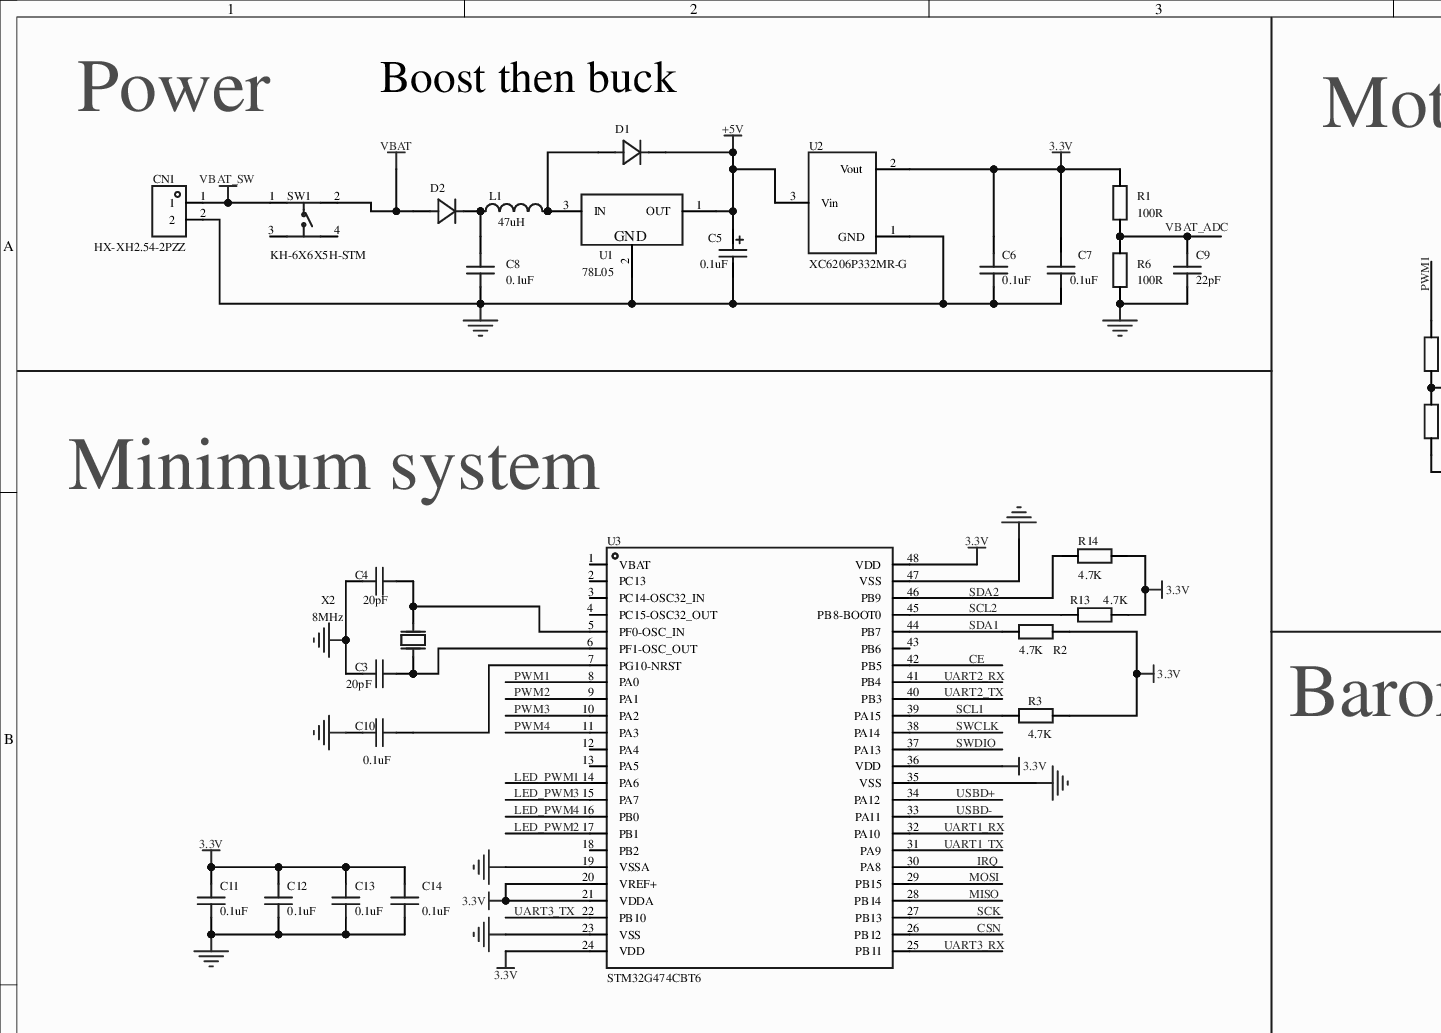
[diagram p0: MISC51791-2.schdoc, top left]
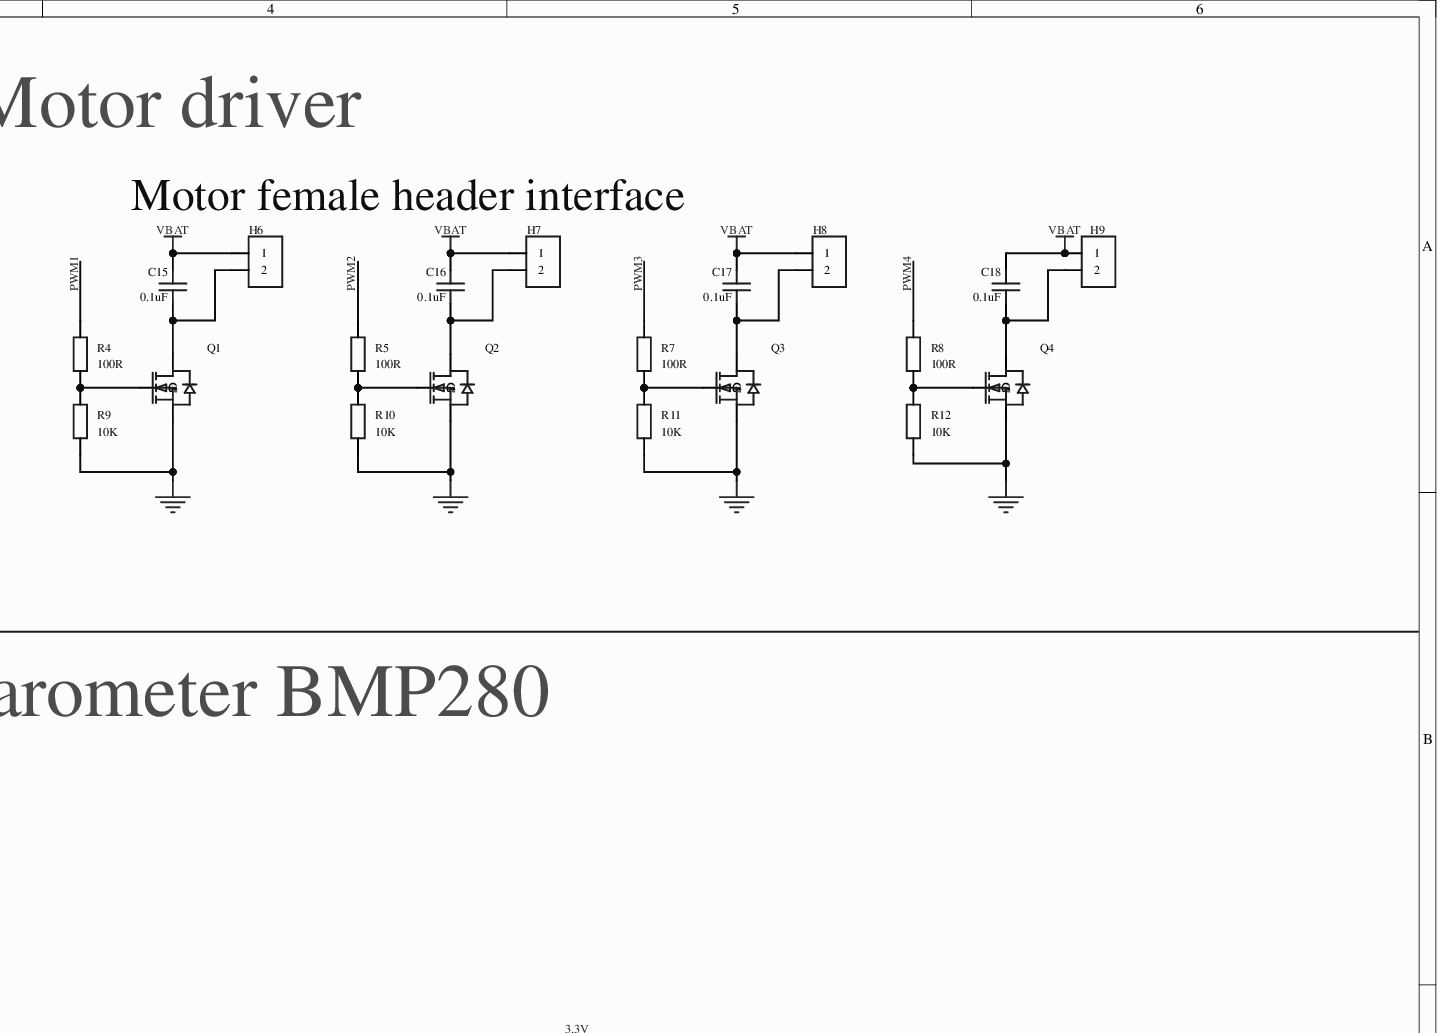
[diagram p1: MISC51791-2.schdoc, top right]
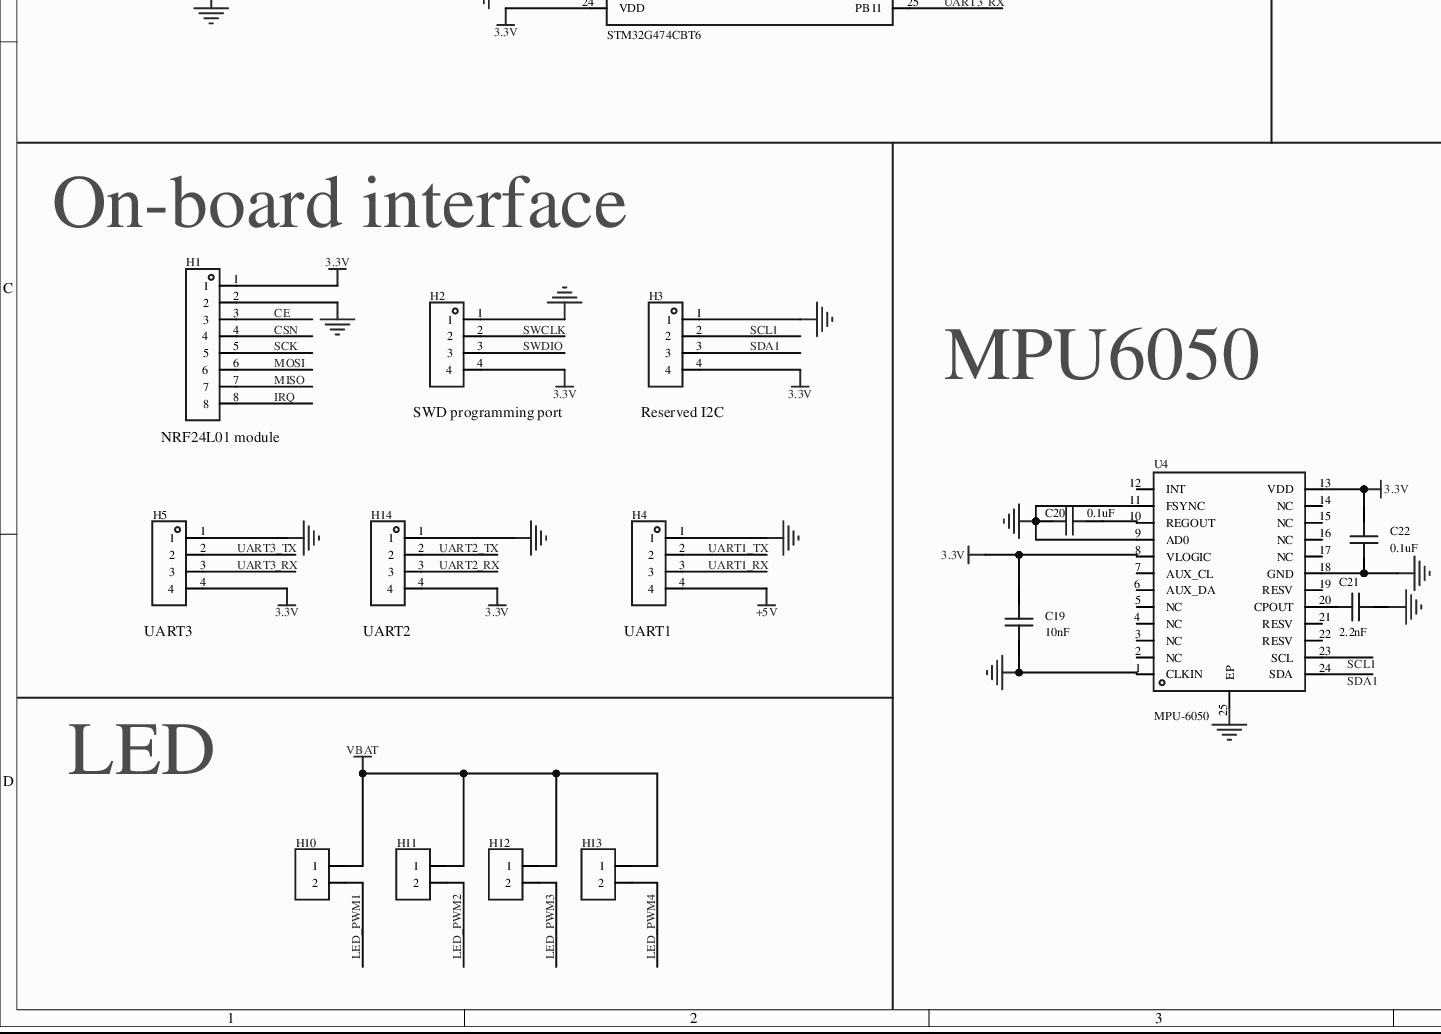
[diagram p2: MISC51791-2.schdoc, bottom left]
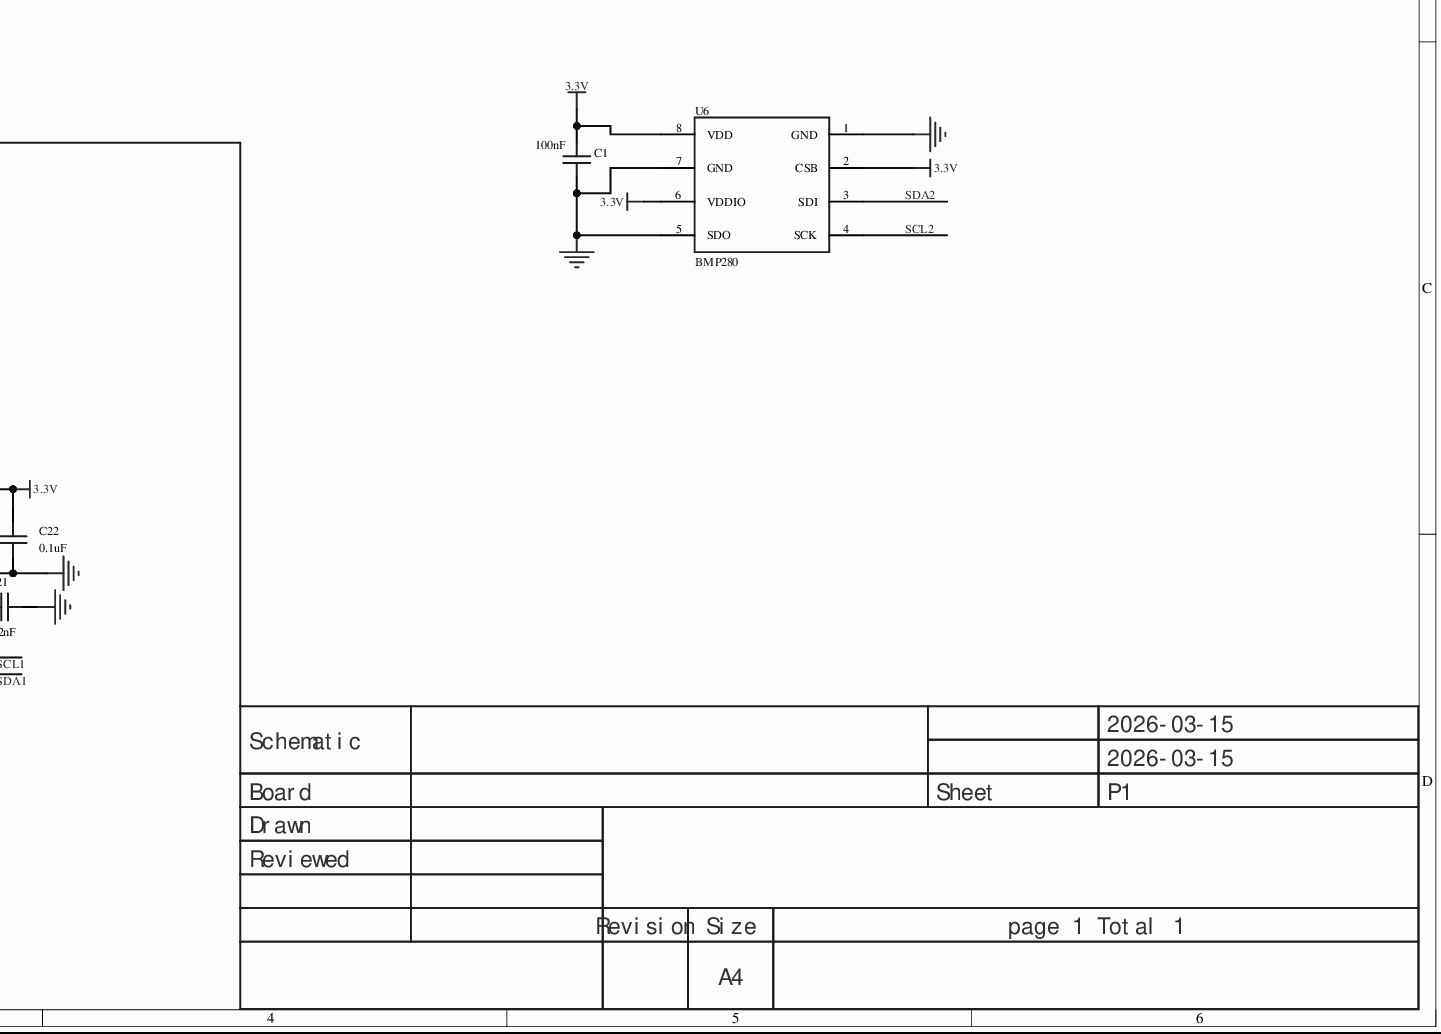
[diagram p3: MISC51791-2.schdoc, bottom right]
# Altium project MISC51791-3.PrjPcb
1 sheet, 64 parts. Net scope: global (net labels, ports and power ports of the same name join across sheets).
Board file: MISC51791.pcbdoc

## Sheet MISC51791-2.schdoc
size 420 x 297 mm; Version: V1.0; @Project Name: MISC51791; @Update Date: 2026-03-15; @Create Date: 2026-03-15; @Board Name: MISC51791; @Create Time: 18:26:02; @Page Count: 1; @Page No: 1; @Schematic Name: MISC51791; @Update Time: 18:26:02; Size: A4

### Parts
C1  100nF  [C0603]
C3  20pF  [C0603]
C4  20pF  [C0603]
C5  0.1uF  [C_Ele_SMD_3x5.4mm]
C6  0.1uF  [C0603]
C7  0.1uF  [C0603]
C8  0.1uF  [C0603]
C9  22pF  [C0603]
C10  0.1uF  [C0603]
C11  0.1uF  [C0603]
C12  0.1uF  [C0603]
C13  0.1uF  [C0603]
C14  0.1uF  [C0603]
C15  0.1uF  [C0603]
C16  0.1uF  [C0603]
C17  0.1uF  [C0603]
C18  0.1uF  [C0603]
C19  10nF  [C0603]
C20  0.1uF  [C0603]
C21  2.2nF  [C0603]
C22  0.1uF  [C0603]
CN1  HX-XH2.54-2PZZ  [CONN-TH_2P-P2.50_HX-2.54MM-2P-ZZ-MS]
D1  (no value)  [DO_1N4007]
D2  (no value)  [DO_1N4007]
H1  (no value)  [HDR-TH_8P-P2.54-V-F-1]
H2  (no value)  [HDR-TH_4P-P2.54-V-F]
H3  (no value)  [HDR-TH_4P-P2.54-V-F]
H4  (no value)  [HDR-TH_4P-P2.54-V-F]
H5  (no value)  [HDR-TH_4P-P2.54-V-F]
H6  (no value)  [HDR-TH_2P-P2.54-V-F]
H7  (no value)  [HDR-TH_2P-P2.54-V-F]
H8  (no value)  [HDR-TH_2P-P2.54-V-F]
H9  (no value)  [HDR-TH_2P-P2.54-V-F]
H10  (no value)  [HDR-TH_2P-P2.54-V-F]
H11  (no value)  [HDR-TH_2P-P2.54-V-F]
H12  (no value)  [HDR-TH_2P-P2.54-V-F]
H13  (no value)  [HDR-TH_2P-P2.54-V-F]
H14  (no value)  [HDR-TH_4P-P2.54-V-F]
L1  47uH  [L0603]
Q1  (no value)  [SOT-23-3_L2.9-W1.3-P1.90-LS2.4-BR]
Q2  (no value)  [SOT-23-3_L2.9-W1.3-P1.90-LS2.4-BR]
Q3  (no value)  [SOT-23-3_L2.9-W1.3-P1.90-LS2.4-BR]
Q4  (no value)  [SOT-23-3_L2.9-W1.3-P1.90-LS2.4-BR]
R1  100R  [R0603]
R2  4.7K  [R0603]
R3  4.7K  [R0603]
R4  100R  [R0603]
R5  100R  [R0603]
R6  100R  [R0603]
R7  100R  [R0603]
R8  100R  [R0603]
R9  10K  [R0603]
R10  10K  [R0603]
R11  10K  [R0603]
R12  10K  [R0603]
R13  4.7K  [R0603]
R14  4.7K  [R0603]
SW1  KH-6X6X5H-STM  [SW-SMD_4P-L6.0-W6.0-P4.50-LS9.0_H5.0]
U1  78L05  [SOT-89-3_L4.5-W2.5-P1.50-LS4.2-BR]
U2  XC6206P332MR-G  [SOT-23-3_L2.9-W1.6-P1.90-LS2.8-BR]
U3  STM32G474CBT6  [LQFP-48_L7.0-W7.0-P0.50-LS9.0-BL]
U4  MPU-6050  [QFN-24_L4.0-W4.0-P0.50-BL-EP2.7]
U6  BMP280  [LGA-8_L2.5-W2.0-P0.65_AMP6127]
X2  8MHz  [CRYSTAL-SMD_L5.0-W3.2]

### Nets
3.3V: C1.2 C6.2 C7.2 C11.2 C12.2 C13.2 C14.2 C19.2 C22.1 H1.1 H2.4 H3.4 H5.4 H14.4 R1.2 R2.2 R3.2 R13.2 R14.2 U2.2(Vout) U3.20(VREF+) U3.21(VDDA) U3.24(VDD) U3.36(VDD) U3.48(VDD) U4.8(VLOGIC) U4.13(VDD) U6.2(CSB) U6.6(VDDIO) U6.8(VDD)
+5V: C5.1 D1.1(K) H4.4 U1.1(OUT) U2.3(Vin)
GND: C1.1 C3.1 C4.1 C5.2 C6.1 C7.1 C8.1 C9.1 C10.1 C11.1 C12.1 C13.1 C14.1 C19.1 C20.1 C21.2 C22.2 CN1.2 H1.2 H2.1 H3.1 H4.1 H5.1 H14.1 Q1.2(S) Q2.2(S) Q3.2(S) Q4.2(S) R6.1 R9.1 R10.1 R11.1 R12.1 U1.2(GND) U2.1(GND) U3.19(VSSA) U3.23(VSS) U3.35(VSS) U3.47(VSS) U4.1(CLKIN) U4.9(AD0) U4.11(FSYNC) U4.18(GND) U4.25(EP) U6.1(GND) U6.5(SDO) U6.7(GND)
VBAT: C15.2 C16.2 C17.2 C18.2 D2.2(A) H6.1 H7.1 H8.1 H9.1 H10.1 H11.1 H12.1 H13.1 SW1.2
VBAT_SW: CN1.1 SW1.1
CE: H1.3 U3.42(PB5)
CSN: H1.4 U3.26(PB12)
IRQ: H1.8 U3.30(PA8)
LED_PWM1: H10.2 U3.14(PA6)
LED_PWM2: H11.2 U3.17(PB1)
LED_PWM3: H12.2 U3.15(PA7)
LED_PWM4: H13.2 U3.16(PB0)
MISO: H1.7 U3.28(PB14)
MOSI: H1.6 U3.29(PB15)
PWM1: R4.2 U3.8(PA0)
PWM2: R5.2 U3.9(PA1)
PWM3: R7.2 U3.10(PA2)
PWM4: R8.2 U3.11(PA3)
SCK: H1.5 U3.27(PB13)
SCL1: H3.2 R3.1 U3.39(PA15) U4.23(SCL)
SCL2: R13.1 U3.45(PB8-BOOT0) U6.4(SCK)
SDA1: H3.3 R2.1 U3.44(PB7) U4.24(SDA)
SDA2: R14.1 U3.46(PB9) U6.3(SDI)
SWCLK: H2.2 U3.38(PA14)
SWDIO: H2.3 U3.37(PA13)
UART1_RX: H4.3 U3.32(PA10)
UART1_TX: H4.2 U3.31(PA9)
UART2_RX: H14.3 U3.41(PB4)
UART2_TX: H14.2 U3.40(PB3)
UART3_RX: H5.3 U3.25(PB11)
UART3_TX: H5.2 U3.22(PB10)
USBD+: U3.34(PA12)
USBD-: U3.33(PA11)
NetC3_2: C3.2 U3.6(PF1-OSC_OUT) X2.1(OSC1)
NetC4_2: C4.2 U3.5(PF0-OSC_IN) X2.2(OSC2)
NetC8_2: C8.2 D2.1(K) L1.1
NetC9_2: C9.2 R1.1 R6.2
NetC10_2: C10.2 U3.7(PG10-NRST)
NetC15_1: C15.1 H6.2 Q1.3(D)
NetC16_1: C16.1 H7.2 Q2.3(D)
NetC17_1: C17.1 H8.2 Q3.3(D)
NetC18_1: C18.1 H9.2 Q4.3(D)
NetC20_2: C20.2 U4.10(REGOUT)
NetC21_1: C21.1 U4.20(CPOUT)
NetD1_2: D1.2(A) L1.2 U1.3(IN)
NetQ1_1: Q1.1(G) R4.1 R9.2
NetQ2_1: Q2.1(G) R5.1 R10.2
NetQ3_1: Q3.1(G) R7.1 R11.2
NetQ4_1: Q4.1(G) R8.1 R12.2

Not connected (* = marked no-connect by the designer): SW1 3* 4*; U3 1(VBAT)* 2(PC13)* 3(PC14-OSC32_IN)* 4(PC15-OSC32_OUT)* 12(PA4)* 13(PA5)* 18(PB2)* 43(PB6)*; U4 2(NC)* 3(NC)* 4(NC)* 5(NC)* 6(AUX_DA)* 7(AUX_CL)* 12(INT)* 14(NC)* 15(NC)* 16(NC)* 17(NC)* 19(RESV)* 21(RESV)* 22(RESV)*

### Notes on the sheet
- Power
- (near D1) Boost then buck
- Motor driver
- Motor female header interface
- Minimum system
- Barometer BMP280
- (near H1) On-board interface
- MPU6050
- (near H1) NRF24L01 module
- (near H2) SWD programming port
- (near H3) Reserved I2C
- (near H5) UART3
- (near H14) UART2
- (near H4) UART1
- LED
- Labels drawn without touching a wire or pin: VBAT_ADC
- 2026-03-15
- Schematic
- Board
- Sheet
- P1
- Drawn
- Reviewed
- Revision
- Size
- A4
- page 1 Total 1

### Library data of the parts
C1 C3 C4 C6-C22 = CAP_0603: Symbol: Capacitance; 3D Model: ac125912035d415993ca9572d50418b10819f05c4eef4c71ace90d822a990e87; 3D Model Transform: 62.992,31.496,0,0,0,0,0,0,0; ConvertToPcb: yes; ModelName: C0603_L1.6-W0.8-H0.8; Device: CAP_0603; Supplier Footprint: 0603; AddInBom: yes; FootprintName: C0603
  C1: Value: 100nF
  C3 C4: Value: 20pF
  C6-C8 C10-C18 C20 C22: Value: 0.1uF
  C9: Value: 22pF
  C19: Value: 10nF
  C21: Value: 2.2nF
C5 = C_Ele_SMD_3x5.4mm: Symbol: CAP; 3D Model: 0132c3d3fdbf4fd987f710a97e7a5b5d; 3D Model Transform: 129.9,149.58,209.06,-90,0,0,0,0,0; AddInBom: yes; ModelName: CAP-SMD_BD3.0-L3.3-W3.3-H5.3; Device: C_Ele_SMD_3x5.4mm; Supplier Footprint: SMD,3x5.4mm; Value: 0.1uF; ConvertToPcb: yes; FootprintName: C_Ele_SMD_3x5.4mm
CN1 = HX-XH2.54-2PZZ: Pin structure: 1x2P; pitch: 2.54mm; mounting: through-hole; reference series: XH; total pins: 2P; rows: 1; pins per row: 2; row spacing: -; rated current: 3A; contact material: brass; contact plating: tin; operating temperature: -25℃~+85℃;; Manufacturer: hanxia(韩下); 3D Model: 1cafe43f43c04794b29c478db770ea2f; 3D Model Transform: 295.275,228.7397,0,0,0,0,0,-19.685,-137.795; Number of PINs Per Row: 2; Voltage Rating: 250V; Plastic Material: PA66; Flame Retardant Rating: UL94V-0; AddInBom: yes; Symbol: HX-XH2.54-2PZZ; Device: HX-XH2.54-2PZZ; LCSC Part Name: 1x2P 间距:2.5mm 直插 系列:XH; Supplier Part: C42391660; Manufacturer Part: HX-XH2.54-2PZZ; Supplier Footprint: 插件,P=2.5mm; JLCPCB Part Class: Extended library; Datasheet: https://item.szlcsc.com/datasheet/HX-XH2.54-2PZZ/44326932.html; Supplier: LCSC; Pins Structure: 1x2P; Pitch: 2.54mm; Mounting Type: Through-hole; Reference Series: XH; Number of Pins: 2P; Number of Rows: 1; Row Spacing: -; Current Rating: 3A; Contact Material: Brass; Contact Plating: Tin; Operating Temperature: -25℃~+85℃; Color: White; ConvertToPcb: yes; FootprintName: CONN-TH_2P-P2.50_HX-2.54MM-2P-ZZ-MS; ModelName: CONN-TH_2P-P2.50_HX-2.54MM-2P-ZZ-MS
D1 D2 = D_1N4007A: AddInBom: yes; ModelId: 6de1e9b71a0d4751b4e9df530304c1a30819f05c4eef4c71ace90d822a990e87; ModelName: DO-41_D2.4-L4.7-P8.70; ModelTransform: 373.9,94.4,232.29,0,0,0,0,0,-140; Symbol: D_1N4007; Device: D_1N4007A; Supplier Footprint: DO-41; ConvertToPcb: yes; FootprintName: DO_1N4007
H1 = HDR-F_2.54_1x8P: Symbol: Header-Female-2.54_1x8; 3D Model: 0f7e4d9227ef4fa08d5469c22cc70cdb0819f05c4eef4c71ace90d822a990e87; 3D Model Transform: 799.99844,100,0,0,0,0,0,0,-118.11; AddInBom: yes; ModelName: HDR-F-2.54_1x8; Device: HDR-F_2.54_1x8P; Supplier Part: C27438; Supplier Footprint: 插件; ConvertToPcb: yes; FootprintName: HDR-TH_8P-P2.54-V-F-1
H2-H5 H14 = HDR-F_2.54_1x4P: Symbol: 2.54-1*4P female; 3D Model: d187812051054f85879fcaa51a310d8e0819f05c4eef4c71ace90d822a990e87; 3D Model Transform: 419.6842,98.464,0,0,0,0,0,0,-118.11; ConvertToPcb: yes; Device: HDR-F_2.54_1x4P; Supplier Part: C2718488; Supplier Footprint: 插件; AddInBom: yes; FootprintName: HDR-TH_4P-P2.54-V-F; ModelName: HDR-TH_4P-P2.54-V-F
H6-H13 = HDR-F_2.54_1x2P: Symbol: Header-Female-2.54_1x2; ConvertToPcb: yes; ModelId: a9450ef445564560a104363b9aacde4e0819f05c4eef4c71ace90d822a990e87; ModelName: HDR-TH_2P-P2.54-F-LI-1X2P; ModelTransform: 215.7476,98.425,0,0,0,0,0,0,-129.921; Device: HDR-F_2.54_1x2P; AddInBom: yes; SupplierPart: C49661; Supplier Footprint: 插件; FootprintName: HDR-TH_2P-P2.54-V-F
L1 = L_0603: Symbol: SDFL1608S100KTF; AddInBom: yes; ModelId: 2bc5ec593d464d6ba9807aec0b5673c20819f05c4eef4c71ace90d822a990e87; ModelName: L0603_L1.6-W0.8-H0.5_BEAD; ModelTransform: 62.992,31.496,0,180,0,0,0.094,0.629,0; Device: L_0603; Value: 47uH; Supplier Footprint: L0603; ConvertToPcb: yes; FootprintName: L0603
Q1-Q4 = AO3400A_N: Type: N-channel; drain-source voltage (Vdss): 30V; continuous drain current (Id): 5.2A; power (Pd): 1W; on-resistance (RDS(on)@Vgs,Id): 35mΩ@10V,5A; threshold voltage (Vgs(th)@Id): 1.5V@250; Symbol: N_MOS; AddInBom: yes; ModelId: c62791f0466c4ae2a892c056b845b0ca0819f05c4eef4c71ace90d822a990e87; ModelName: SOT-23-3P_L2.9-W1.3-H1.0-LS2.4-P0.95; ModelTransform: 98.425,114.173,0,180,0,0,0.0005,-0.0005,0; Device: AO3400A_N; Supplier Footprint: SOT-23; ConvertToPcb: yes; FootprintName: SOT-23-3_L2.9-W1.3-P1.90-LS2.4-BR; SupplierPart: C700953
R1-R14 = Res_0603: Symbol: Resistor; 3D Model: fc143cca1e79419f9cd78b61e9279f08; 3D Model Transform: 31.8897,63.7794,0,90,0,0,0,0,0; ConvertToPcb: yes; Device: Res_0603; Supplier Footprint: 0603; AddInBom: yes; FootprintName: R0603; ModelName: R0603
  R1 R4-R8: Value: 100R
  R2 R3 R13 R14: Value: 4.7K
  R9-R12: Value: 10K
SW1 = KH-6X6X5H-STM: Circuit structure: SPST; button shape: round button; mounting: surface mount; switch length: 6mm; switch width: 6mm; switch height: 5mm; with bracket: without bracket; contact current: 50mA; rated voltage: 12V; service life: 8万 cycles;; Manufacturer: kinghelm(金航标); AddInBom: yes; ModelId: 46371efb35684031937580a0045530ec0819f05c4eef4c71ace90d822a990e87; ModelTransform: 354.33,236.25937,0,0,0,0,0,0,0; Actuator/Cap Color: Black; Symbol: KH-6X6X5H-STM; Device: KH-6X6X5H-STM; LCSC Part Name: 6*6*5mm 立贴 轻触开关; SupplierPart: C2837531; ManufacturerPart: KH-6X6X5H-STM; Supplier Footprint: SMD-4P,6x6mm; JLCPCB Part Class: Extended Part; Datasheet: https://item.szlcsc.com/datasheet/KH-6X6X5H-STM/3009601.html; Supplier: LCSC; ConvertToPcb: yes; FootprintName: SW-SMD_4P-L6.0-W6.0-P4.50-LS9.0_H5.0; ModelName: SW-SMD_4P-L6.0-W6.0-P4.50-LS9.0_H5.0; Circuit: SPST; Actuator Style: Round button; Mounting Type: Surface mount; Length: 6mm; Width: 6mm; Switch Height: 5mm; with Bracket: Without bracket; Contact Current: 50mA; Voltage Rating: 12V; Termination Style: Gull-wing; Life: 8万 cycles
U1 = 78L05_C347258: Output type: fixed; operating voltage: 30V; output voltage: 5V; output current: 100mA; ripple rejection (PSRR): 49dB@(120Hz); output polarity: positive;; Manufacturer: UMW(友台半导体); Symbol: UMW78L05; AddInBom: yes; ModelId: 6db690b7897d4d18a30d90c1b89525ee0819f05c4eef4c71ace90d822a990e87; ModelName: SOT-89-3_L4.3-W2.5-H1.6-LS4.1-P1.50; ModelTransform: 161.417,169.291,0,180,0,0,-11.808,0,0; Voltage Dropout: 1.7V; standby current: 2mA; Noise: 40uV; Number of Outputs: 1; Device: 78L05_C347258; LCSC Part Name: 5V 100mA 30V; SupplierPart: C347258; ManufacturerPart: 78L05; Supplier Footprint: SOT-89-3; JLCPCB Part Class: Extended Part; Datasheet: https://item.szlcsc.com/datasheet/78L05/323918.html; Supplier: LCSC; ConvertToPcb: yes; FootprintName: SOT-89-3_L4.5-W2.5-P1.50-LS4.2-BR; Output Type: Fixed; Voltage - Supply: 30V; Output Voltage: 5V; Output Current: 100mA; Power Supply Rejection Ratio (PSRR): 49dB@(120Hz); Features: Overheat protection; short-circuit protection; Operating Temperature: -20℃~+120℃@(Tj); Output Configuration: Positive
U2 = XC6206P332MR-G_C5446: Output type: fixed; operating voltage: 6V; output voltage: 3.3V; output current: 200mA; ripple rejection (PSRR): -; output polarity: positive;; Manufacturer: TOREX(特瑞仕); AddInBom: yes; ModelId: 89cb27a44ab2466697082bb9fd73a7d00819f05c4eef4c71ace90d822a990e87; ModelName: SOT-23-3L_L2.9-W1.6-H1.1-LS2.8-P0.95; ModelTransform: 114.173,110.236,0,90,0,0,0,0,0; standby current: 1uA; Number of Outputs: 1; Symbol: XC6206P332MR; Device: XC6206P332MR-G_C5446; LCSC Part Name: 3.3V 200mA 6V; SupplierPart: C5446; ManufacturerPart: XC6206P332MR-G; Supplier Footprint: SOT-23-3L; JLCPCB Part Class: Basic Part; Datasheet: https://item.szlcsc.com/datasheet/XC6206P332MR-G/5896.html; Supplier: LCSC; ConvertToPcb: yes; FootprintName: SOT-23-3_L2.9-W1.6-P1.90-LS2.8-BR; Output Type: Fixed; Voltage - Supply: 6V; Output Voltage: 3.3V; Output Current: 200mA; Power Supply Rejection Ratio (PSRR): -; Voltage Dropout: -; Noise: -; Features: Overcurrent protection; Operating Temperature: -40℃~+85℃@(Ta); Output Configuration: Positive
U3 = STM32G474CBT6: CPU core: ARM Cortex-M4F; max CPU frequency: 170MHz; CPU bits: 32 Bit;; Manufacturer: ST(意法半导体); AddInBom: yes; ModelId: 093be70396ff421eb2cdb946d5311efc0819f05c4eef4c71ace90d822a990e87; ModelName: LQFP-48_L7.0-W7.0-H1.4-LS9.0-P0.50; ModelTransform: 354.331,354.331,0,0,0,0,0,0,0; Core Size: 32 Bit; Program Storage Size: 128KB; Program Memory Type: FLASH; Number of I/O: 38; ADC (Bit): 12bit; Oscillator Type: Built-in; Voltage - Supply: 1.71V~3.6V; Symbol: STM32G474CBT6; Device: STM32G474CBT6; LCSC Part Name: Arm Cortex-M4 32位MCU+FPU，170 MHz/213 DMIPS，128 KB SRAM，丰富的模拟功能、数学加速器，184 ps 12通道高分辨率定时器; SupplierPart: C730123; ManufacturerPart: STM32G474CBT6; Supplier Footprint: LQFP-48(7x7); JLCPCB Part Class: Extended Part; Datasheet: https://item.szlcsc.com/datasheet/STM32G474CBT6/778078.html; Supplier: LCSC; ConvertToPcb: yes; FootprintName: LQFP-48_L7.0-W7.0-P0.50-LS9.0-BL; CPU Core: ARM Cortex-M4F; CPU Maximum Speed: 170MHz; RAM Size: 128KB; EEPROM: -; DAC (Bit): 12bit; Operating Temperature: -40℃~+85℃
U4 = MPU-6050: Sensor type: accelerometer and gyroscope;; Manufacturer: TDK InvenSense(应美盛); Symbol: MPU-6050_C24112; AddInBom: yes; ModelId: 3147e748bde04e038f0f2a42301e48160819f05c4eef4c71ace90d822a990e87; ModelTransform: 158.267,158.267,0,0,0,0,0,0,0; Device: MPU-6050; LCSC Part Name: MPU-6050; SupplierPart: C24112; ManufacturerPart: MPU-6050; Supplier Footprint: QFN-24-EP(4x4); JLCPCB Part Class: Extended Part; Datasheet: https://item.szlcsc.com/datasheet/MPU-6050/24852.html; Supplier: LCSC; ConvertToPcb: yes; FootprintName: QFN-24_L4.0-W4.0-P0.50-BL-EP2.7; ModelName: QFN-24_L4.0-W4.0-P0.50-BL-EP2.7; Sensor Type: Accelerometer and gyroscope; Operating Temperature: -40℃~+85℃
U6 = BMP280: Pressure range: 30Kpa~1.1bar; interface type: SPI; I2C;; Manufacturer: Bosch(博世); AddInBom: yes; ModelId: 6ee05a37397b45cc95a0ccf37ae682e30819f05c4eef4c71ace90d822a990e87; ModelTransform: 78.74,98.425,0,0,0,0,0,0,0; Voltage - Supply: 1.71V~3.6V; Standby Current: 300nA; Absolute Accuracy: 1hpa; Relative Accuracy: 0.12hpa; Temperature Coefficient of Offset(TCO): 1.5pa/K; Symbol: BMP280; Device: BMP280; LCSC Part Name: BMP280; SupplierPart: C83291; ManufacturerPart: BMP280; Supplier Footprint: LGA-8(2x2.5); JLCPCB Part Class: Extended Part; Datasheet: https://item.szlcsc.com/datasheet/BMP280/84455.html; Supplier: LCSC; ConvertToPcb: yes; FootprintName: LGA-8_L2.5-W2.0-P0.65_AMP6127; ModelName: LGA-8_L2.5-W2.0-P0.65_AMP6127; Interface: SPI; I2C; Operating Temperature: -40℃~+85℃
X2 = X50328MSB2GI: Crystal type: SMD crystal; frequency: 8MHz; frequency tolerance at room temperature: ±10ppm; load capacitance: 20pF; frequency stability: ±20ppm;; Manufacturer: YXC(扬兴晶振); AddInBom: yes; ModelId: d7c39c66443246ff83c2003c1e1eb6f10819f05c4eef4c71ace90d822a990e87; ModelTransform: 196.85,125.984,0,0,0,0,0,0,0; Symbol: X50328MSB2GI; Device: X50328MSB2GI; LCSC Part Name: YSX530GA 8MHZ 2P 5032 20PF ±10PPM -40~85℃ (±20PPM); SupplierPart: C115962; ManufacturerPart: X50328MSB2GI; Supplier Footprint: SMD5032-2P; JLCPCB Part Class: Basic Part; Datasheet: https://item.szlcsc.com/datasheet/X50328MSB2GI/117214.html; Supplier: LCSC; ConvertToPcb: yes; FootprintName: CRYSTAL-SMD_L5.0-W3.2; ModelName: CRYSTAL-SMD_L5.0-W3.2; Type: SMD crystal; Value: 8MHz; Normal temperature Frequency Tolerance: ±10ppm; Load Capacitance: 20pF; Frequency Stability: ±20ppm; Operating Temperature: -40℃~+85℃